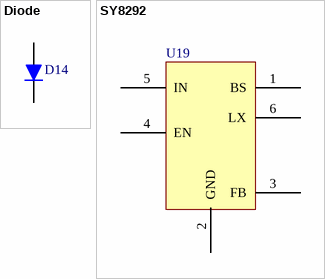
[diagram p0: symbols Diode to SY8292]
# Altium schematic symbol library MISC86294-42.SchLib: 2 symbols
Pins are listed as number, name and electrical type; pins without a type are passive.


## Diode
designator D14
Diode template
pins: 1 K, 2 A

## SY8292
designator U19
5-40V,2A,asynchronous
footprint SOT-23-6_L2.9-W1.6
pins: 1 BS, 2 GND, 3 FB, 4 EN, 5 IN, 6 LX